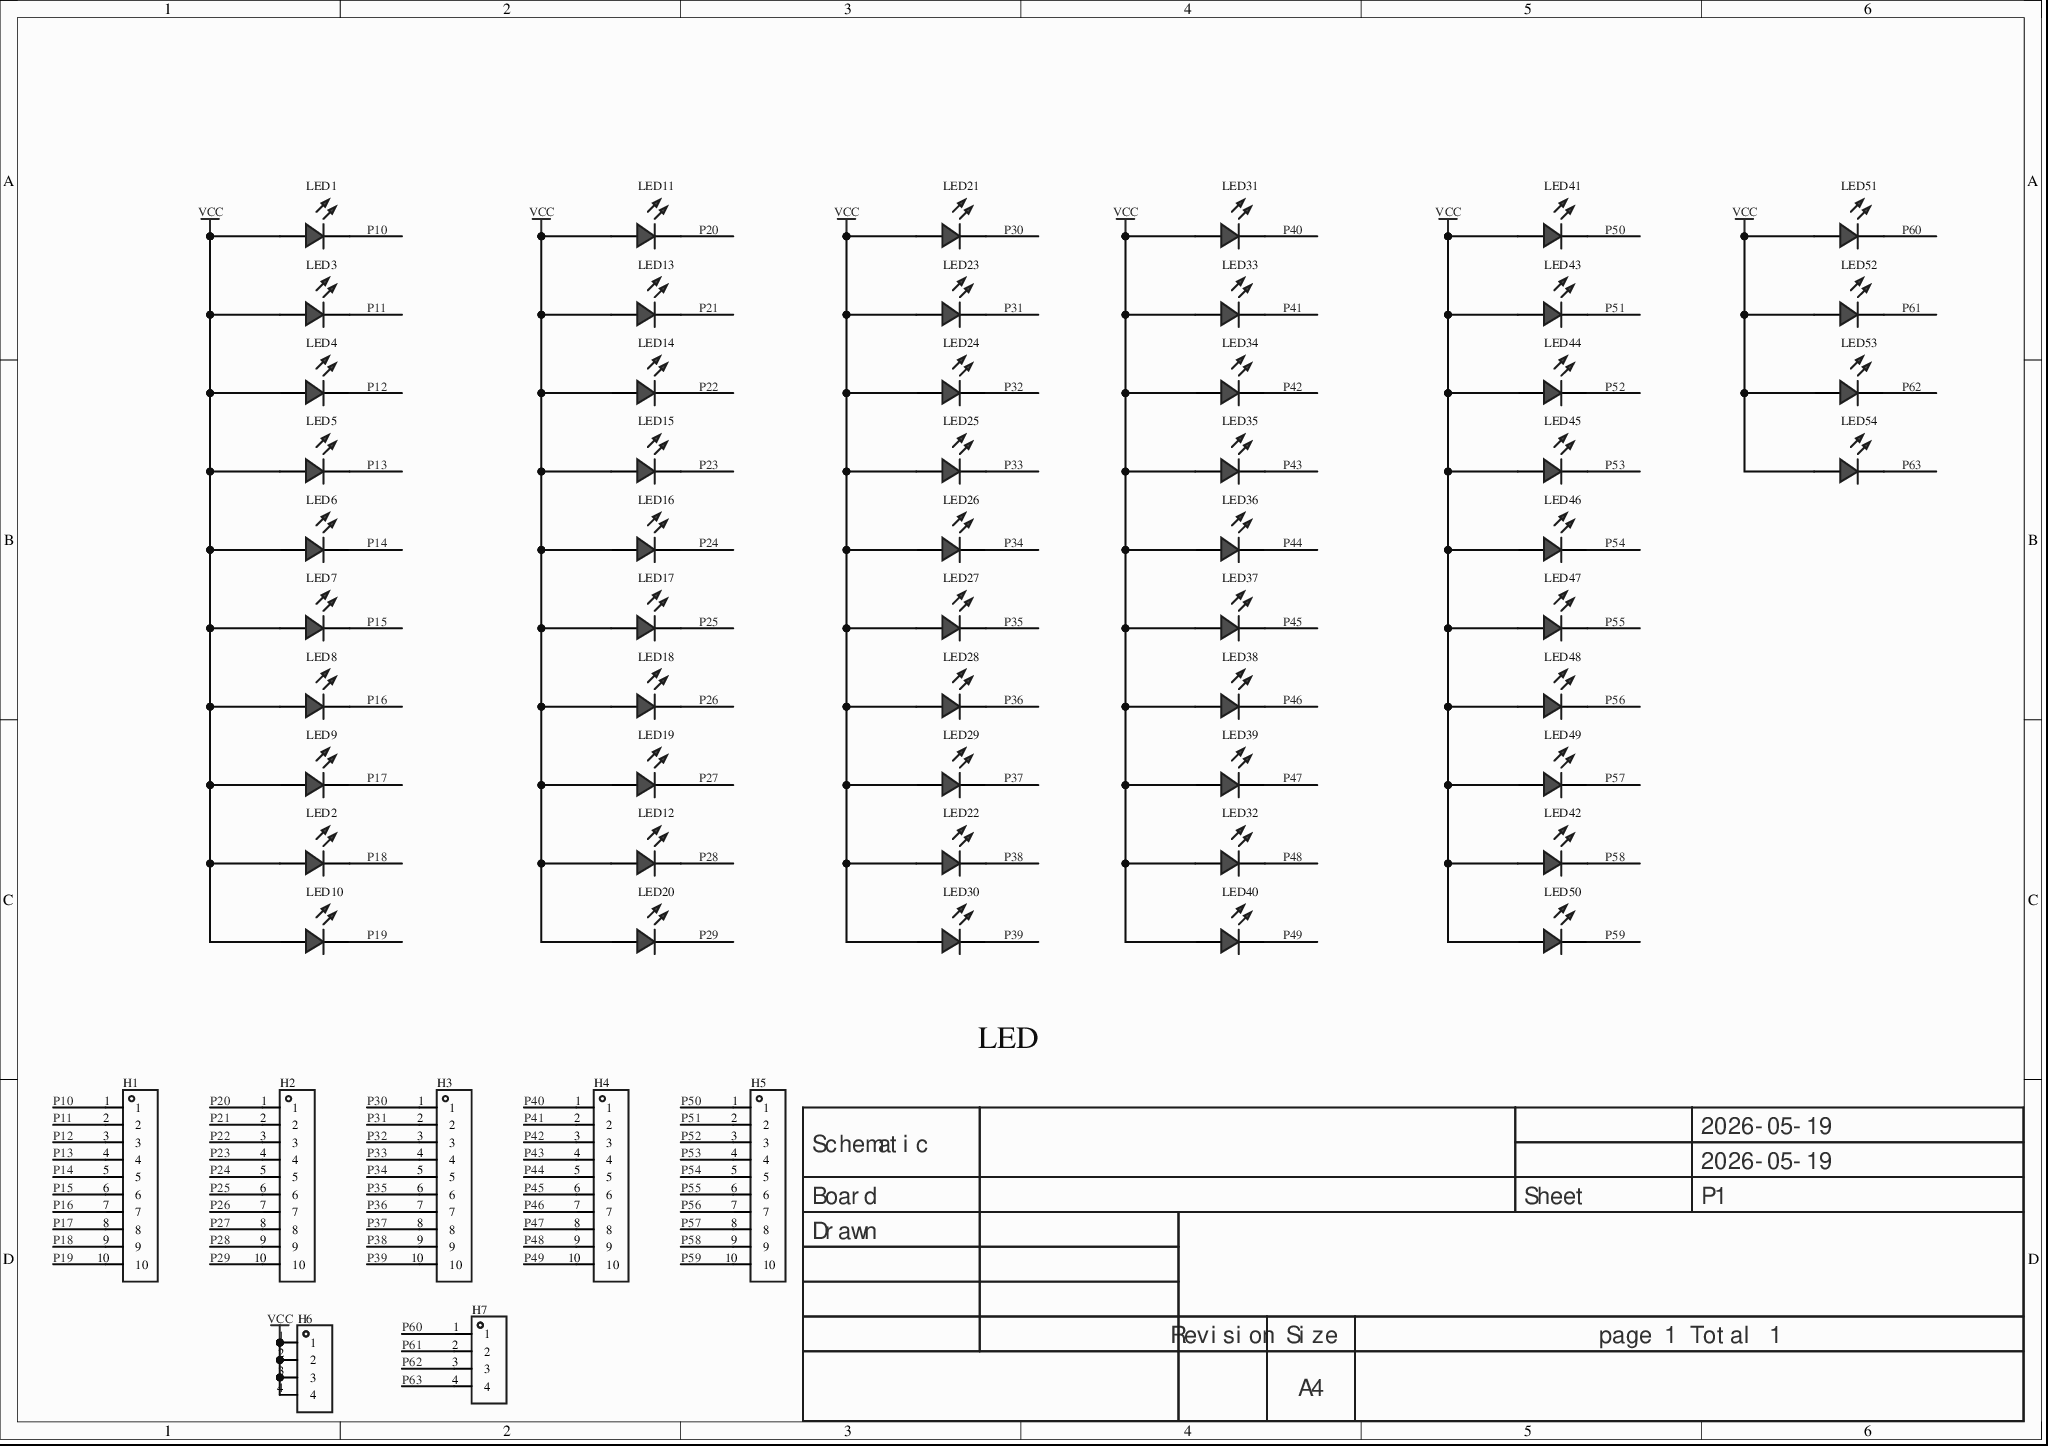
[diagram p0: MISC89091-3.schdoc]
# Altium project MISC89091-2.PrjPcb
1 sheet, 61 parts. Net scope: global (net labels, ports and power ports of the same name join across sheets).
Board file: MISC89091.pcbdoc

## Sheet MISC89091-3.schdoc
size 297 x 209 mm; Version: V1.0; @Project Name: MISC89091; @Update Date: 2026-05-19; @Create Date: 2026-05-19; @Board Name: MISC89091; @Create Time: 22:31:37; @Page Count: 1; @Page No: 1; @Schematic Name: MISC89091; @Update Time: 22:31:37; Size: A4

### Parts
H1  (no value)  [HDR-TH_10P-P2.54-V-F]
H2  (no value)  [HDR-TH_10P-P2.54-V-F]
H3  (no value)  [HDR-TH_10P-P2.54-V-F]
H4  (no value)  [HDR-TH_10P-P2.54-V-F]
H5  (no value)  [HDR-TH_10P-P2.54-V-F]
H6  (no value)  [HDR-TH_4P-P2.54-V-F]
H7  (no value)  [HDR-TH_4P-P2.54-V-F]
LED1  (no value)  [LED_TH-3mm]
LED2  (no value)  [LED_TH-3mm]
LED3  (no value)  [LED_TH-3mm]
LED4  (no value)  [LED_TH-3mm]
LED5  (no value)  [LED_TH-3mm]
LED6  (no value)  [LED_TH-3mm]
LED7  (no value)  [LED_TH-3mm]
LED8  (no value)  [LED_TH-3mm]
LED9  (no value)  [LED_TH-3mm]
LED10  (no value)  [LED_TH-3mm]
LED11  (no value)  [LED_TH-3mm]
LED12  (no value)  [LED_TH-3mm]
LED13  (no value)  [LED_TH-3mm]
LED14  (no value)  [LED_TH-3mm]
LED15  (no value)  [LED_TH-3mm]
LED16  (no value)  [LED_TH-3mm]
LED17  (no value)  [LED_TH-3mm]
LED18  (no value)  [LED_TH-3mm]
LED19  (no value)  [LED_TH-3mm]
LED20  (no value)  [LED_TH-3mm]
LED21  (no value)  [LED_TH-3mm]
LED22  (no value)  [LED_TH-3mm]
LED23  (no value)  [LED_TH-3mm]
LED24  (no value)  [LED_TH-3mm]
LED25  (no value)  [LED_TH-3mm]
LED26  (no value)  [LED_TH-3mm]
LED27  (no value)  [LED_TH-3mm]
LED28  (no value)  [LED_TH-3mm]
LED29  (no value)  [LED_TH-3mm]
LED30  (no value)  [LED_TH-3mm]
LED31  (no value)  [LED_TH-3mm]
LED32  (no value)  [LED_TH-3mm]
LED33  (no value)  [LED_TH-3mm]
LED34  (no value)  [LED_TH-3mm]
LED35  (no value)  [LED_TH-3mm]
LED36  (no value)  [LED_TH-3mm]
LED37  (no value)  [LED_TH-3mm]
LED38  (no value)  [LED_TH-3mm]
LED39  (no value)  [LED_TH-3mm]
LED40  (no value)  [LED_TH-3mm]
LED41  (no value)  [LED_TH-3mm]
LED42  (no value)  [LED_TH-3mm]
LED43  (no value)  [LED_TH-3mm]
LED44  (no value)  [LED_TH-3mm]
LED45  (no value)  [LED_TH-3mm]
LED46  (no value)  [LED_TH-3mm]
LED47  (no value)  [LED_TH-3mm]
LED48  (no value)  [LED_TH-3mm]
LED49  (no value)  [LED_TH-3mm]
LED50  (no value)  [LED_TH-3mm]
LED51  (no value)  [LED_TH-3mm]
LED52  (no value)  [LED_TH-3mm]
LED53  (no value)  [LED_TH-3mm]
LED54  (no value)  [LED_TH-3mm]

### Nets
VCC: H6.1 H6.2 H6.3 H6.4 LED1.1(C) LED2.1(C) LED3.1(C) LED4.1(C) LED5.1(C) LED6.1(C) LED7.1(C) LED8.1(C) LED9.1(C) LED10.1(C) LED11.1(C) LED12.1(C) LED13.1(C) LED14.1(C) LED15.1(C) LED16.1(C) LED17.1(C) LED18.1(C) LED19.1(C) LED20.1(C) LED21.1(C) LED22.1(C) LED23.1(C) LED24.1(C) LED25.1(C) LED26.1(C) LED27.1(C) LED28.1(C) LED29.1(C) LED30.1(C) LED31.1(C) LED32.1(C) LED33.1(C) LED34.1(C) LED35.1(C) LED36.1(C) LED37.1(C) LED38.1(C) LED39.1(C) LED40.1(C) LED41.1(C) LED42.1(C) LED43.1(C) LED44.1(C) LED45.1(C) LED46.1(C) LED47.1(C) LED48.1(C) LED49.1(C) LED50.1(C) LED51.1(C) LED52.1(C) LED53.1(C) LED54.1(C)
P10: H1.1 LED1.2(A)
P11: H1.2 LED3.2(A)
P12: H1.3 LED4.2(A)
P13: H1.4 LED5.2(A)
P14: H1.5 LED6.2(A)
P15: H1.6 LED7.2(A)
P16: H1.7 LED8.2(A)
P17: H1.8 LED9.2(A)
P18: H1.9 LED2.2(A)
P19: H1.10 LED10.2(A)
P20: H2.1 LED11.2(A)
P21: H2.2 LED13.2(A)
P22: H2.3 LED14.2(A)
P23: H2.4 LED15.2(A)
P24: H2.5 LED16.2(A)
P25: H2.6 LED17.2(A)
P26: H2.7 LED18.2(A)
P27: H2.8 LED19.2(A)
P28: H2.9 LED12.2(A)
P29: H2.10 LED20.2(A)
P30: H3.1 LED21.2(A)
P31: H3.2 LED23.2(A)
P32: H3.3 LED24.2(A)
P33: H3.4 LED25.2(A)
P34: H3.5 LED26.2(A)
P35: H3.6 LED27.2(A)
P36: H3.7 LED28.2(A)
P37: H3.8 LED29.2(A)
P38: H3.9 LED22.2(A)
P39: H3.10 LED30.2(A)
P40: H4.1 LED31.2(A)
P41: H4.2 LED33.2(A)
P42: H4.3 LED34.2(A)
P43: H4.4 LED35.2(A)
P44: H4.5 LED36.2(A)
P45: H4.6 LED37.2(A)
P46: H4.7 LED38.2(A)
P47: H4.8 LED39.2(A)
P48: H4.9 LED32.2(A)
P49: H4.10 LED40.2(A)
P50: H5.1 LED41.2(A)
P51: H5.2 LED43.2(A)
P52: H5.3 LED44.2(A)
P53: H5.4 LED45.2(A)
P54: H5.5 LED46.2(A)
P55: H5.6 LED47.2(A)
P56: H5.7 LED48.2(A)
P57: H5.8 LED49.2(A)
P58: H5.9 LED42.2(A)
P59: H5.10 LED50.2(A)
P60: H7.1 LED51.2(A)
P61: H7.2 LED52.2(A)
P62: H7.3 LED53.2(A)
P63: H7.4 LED54.2(A)

### Notes on the sheet
- LED
- 2026-05-19
- Schematic
- Board
- Sheet
- P1
- Drawn
- Revision
- Size
- A4
- page 1 Total 1

### Library data of the parts
H1-H5 = HDR-F_2.54_1x10P: Symbol: X5511FV-10-C70D30-1000; AddInBom: yes; ModelId: 08a5ee31ec6747838a696d2ac093ffa40819f05c4eef4c71ace90d822a990e87; ModelName: HDR-TH_10P-P2.54-F-LI-1X10P; ModelTransform: 1009.87987,100,0,0,0,0,0,0,-125.984; Device: HDR-F_2.54_1x10P; ConvertToPcb: yes; FootprintName: HDR-TH_10P-P2.54-V-F; SupplierPart: C2684744; Supplier Footprint: 插件
H6 H7 = HDR-F_2.54_1x4P: Symbol: 2.54-1*4P male; ConvertToPcb: yes; ModelId: d187812051054f85879fcaa51a310d8e0819f05c4eef4c71ace90d822a990e87; ModelTransform: 419.6842,98.464,0,0,0,0,0,0,-118.11; Device: HDR-F_2.54_1x4P; AddInBom: yes; SupplierPart: C2718488; Supplier Footprint: 插件; FootprintName: HDR-TH_4P-P2.54-V-F; ModelName: HDR-TH_4P-P2.54-V-F
LED1-LED54 = LED_TH-R_3mm: 3D Model: a497c992633541038a38947cdc58012f0819f05c4eef4c71ace90d822a990e87; 3D Model Transform: 141.274,153.327,0,0,0,0,-5.984,0,-137.795; ConvertToPcb: yes; ModelName: LED-TH-3mm_R; Symbol: LED_TH-R; Device: LED_TH-R_3mm; Supplier Footprint: 插件; AddInBom: yes; FootprintName: LED_TH-3mm